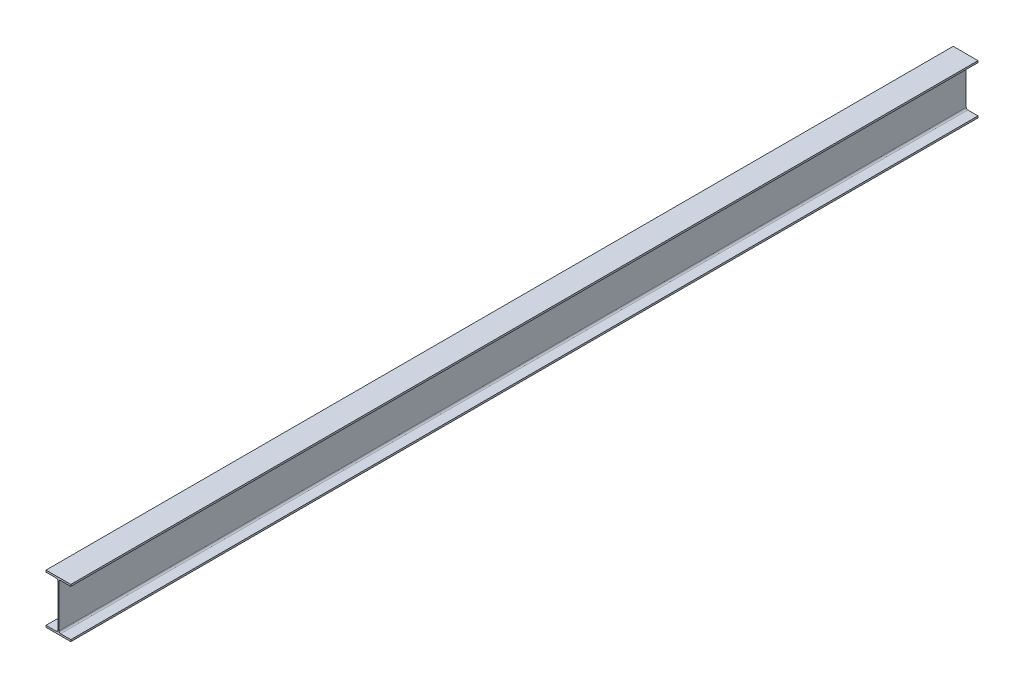
from build123d import *

# Parameters (mm, degrees)
BOSS_EXTRUDE1_DEPTH = 4570


with BuildPart() as part:
    # Sketch1 → Boss-Extrude1 (new body)
    with BuildSketch(Plane.XY):
        with BuildLine():
            Line((62.5, 0), (-62.5, 0))
            Line((-62.5, 0), (-62.5, 9))
            Line((-62.5, 9), (-11, 9))
            ThreePointArc((-11, 9), (-5.343145751, 11.343145751), (-3, 17))
            Line((-3, 17), (-3, 233))
            ThreePointArc((-3, 233), (-5.343145751, 238.656854249), (-11, 241))
            Line((-11, 241), (-62.5, 241))
            Line((-62.5, 241), (-62.5, 250))
            Line((-62.5, 250), (62.5, 250))
            Line((62.5, 250), (62.5, 241))
            Line((62.5, 241), (11, 241))
            ThreePointArc((11, 241), (5.343145751, 238.656854249), (3, 233))
            Line((3, 233), (3, 17))
            ThreePointArc((3, 17), (5.343145751, 11.343145751), (11, 9))
            Line((11, 9), (62.5, 9))
            Line((62.5, 9), (62.5, 0))
        make_face()
    extrude(amount=BOSS_EXTRUDE1_DEPTH)


solid = part.part
